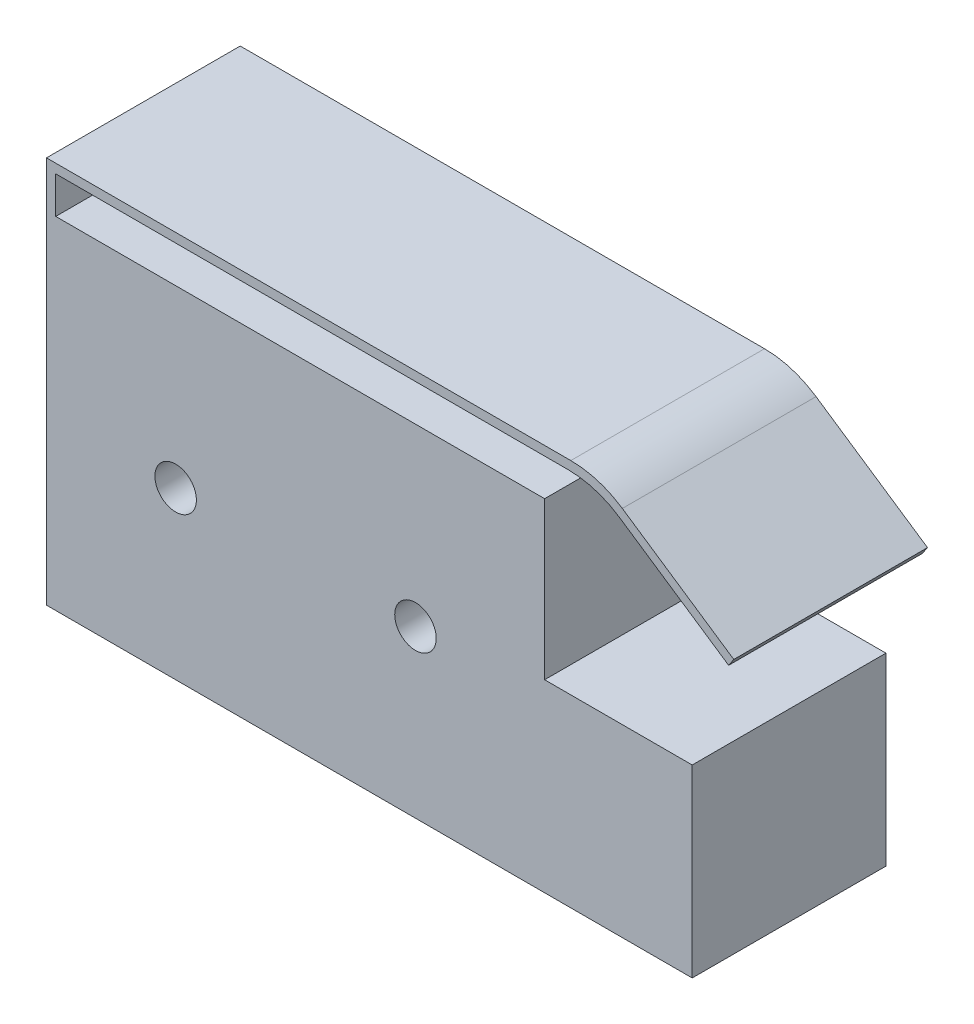
SolidWorks part; units mm, degrees
ref_plane "前视基准面" through (0, 0, 0) normal (0, 0, 1) x (1, 0, 0)
ref_plane "上视基准面" through (0, 0, 0) normal (0, 1, 0) x (1, 0, 0)
ref_plane "右视基准面" through (0, 0, 0) normal (1, 0, 0) x (0, 0, -1)
sketch "草图1" plane through (0, 0, 0) normal (0, 0, 1) x (1, 0, 0)
  line L1 (0, 0) -> (70, 0)
  line L2 (0, 0) -> (0, 37)
  line L3 (0, 37) -> (54, 37)
  line L4 (54, 20) -> (54, 37)
  line L7 (54, 20) -> (70, 20)
  line L8 (70, 0) -> (70, 20)
  circle A0 centre (14, 18) radius 2.25
  circle A1 centre (40, 18) radius 2.25
  dimension "D5" = 4.5
  dimension "D6" = 4.5
  dimension "D7" = 14
  dimension "D8" = 26
  dimension "D9" = 18
  dimension "D10" = 18
  dimension "D1" = 54
  dimension "D2" = 37
  dimension "D3" = 16
  dimension "D4" = 20
extrude "凸台-拉伸1" add sketch "草图1" along normal blind 21
sketch "草图2" plane through (0, 0, 21) normal (0, 0, 1) x (1, 0, 0)
  line L0 (62.4237, 40.2951) -> (74.5062, 32.1603)
  line L1 (0, 37) -> (1, 37)
  line L2 (0, 37) -> (0, 42)
  line L3 (62.1184, 39.2951) -> (73.9477, 31.3307)
  line L4 (1, 37) -> (1, 41)
  line L5 (0, 42) -> (56.8388, 42)
  line L6 (74.5062, 32.1603) -> (73.9477, 31.3307)
  line L7 (1, 41) -> (56.5335, 41)
  line L9 (54, 37) -> (0, 37) construction
  arc A0 (62.4237, 40.2951) -> (56.8388, 42) centre (56.8388, 32) ccw
  arc A1 (62.1184, 39.2951) -> (56.5335, 41) centre (56.5335, 31) ccw
  dimension "D6" = 10
  dimension "D1" = 1
  dimension "D2" = 1
  dimension "D3" = 90
  dimension "D4" = 1
  dimension "D5" = 5
extrude "凸台-拉伸3" add sketch "草图2" against normal up to surface (21 mm away) up to face at (16.25, 18, 0)
